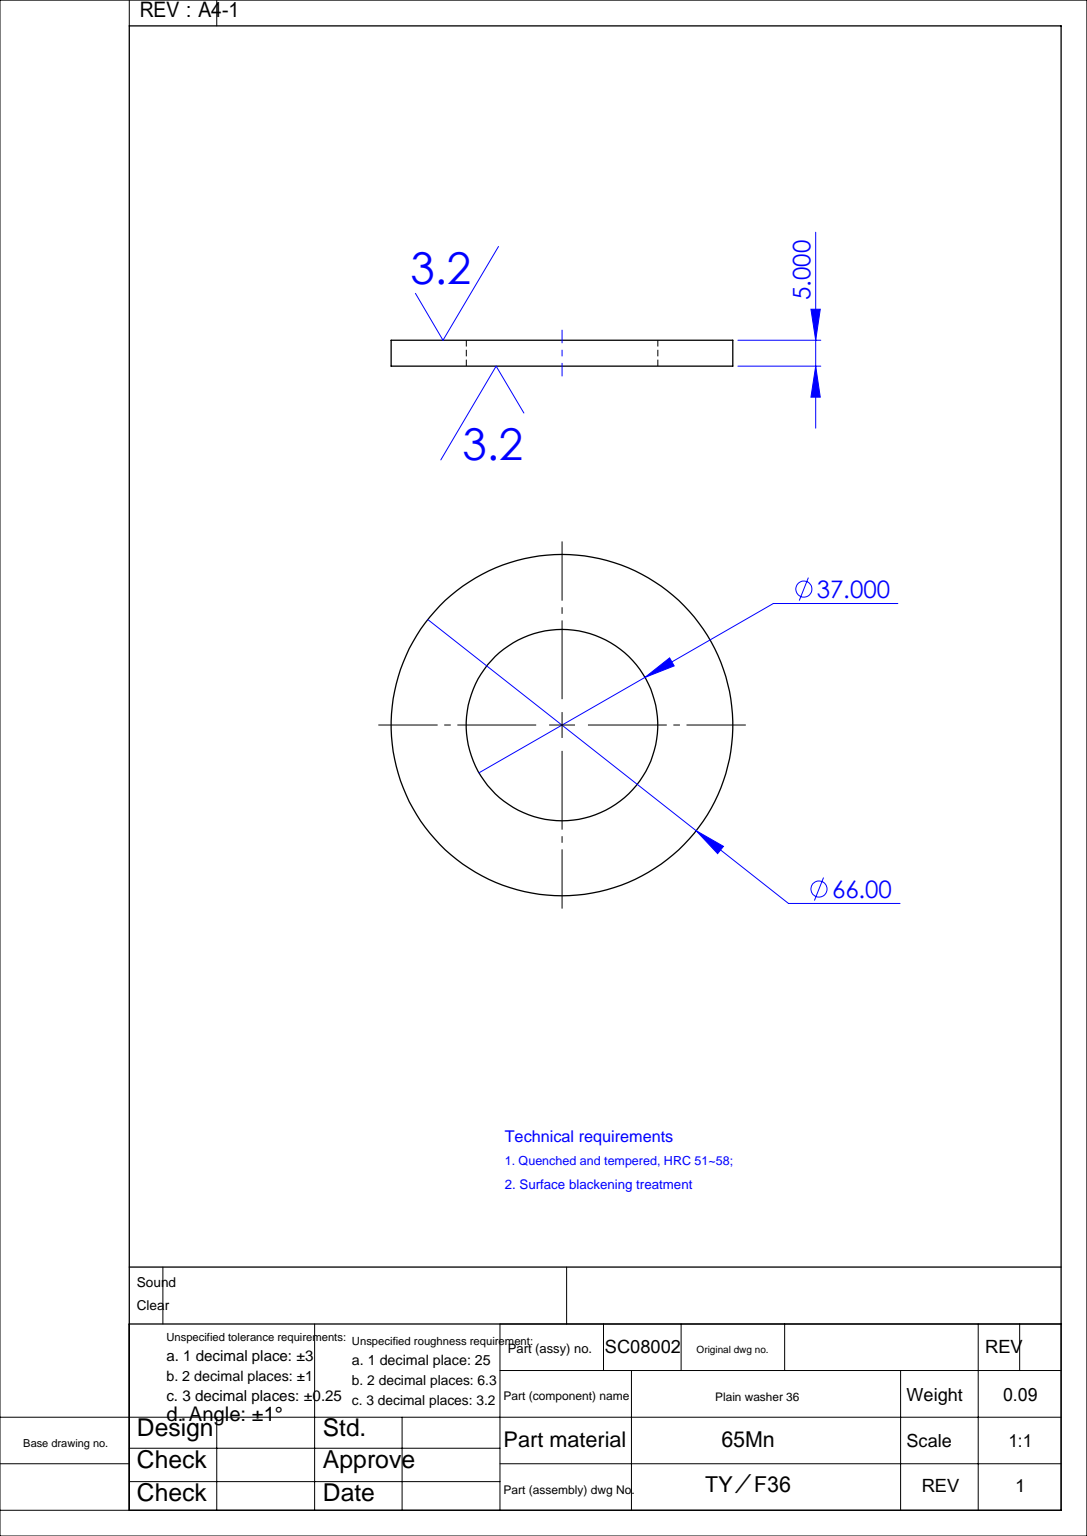
SolidWorks part; units mm, degrees
material "65Mn"
ref_plane "Plane1" through (0, 0, 0) normal (0, 0, 1) x (1, 0, 0)
ref_plane "Plane2" through (0, 0, 0) normal (0, 1, 0) x (1, 0, 0)
ref_plane "Plane3" through (0, 0, 0) normal (1, 0, 0) x (0, 0, -1)
sketch "Dimension sketch" plane through (0, 0, 0) normal (0, 0, 1) x (1, 0, 0)
  line L0 (0, 0) -> (9.1, 0)
  point P3 (1, 0)
  point P4 (10, 0)
  point P5 (5.5, 0)
  dimension "h" = 1
  dimension "d2" = 10
  dimension "d1" = 5.5
sketch "Sketch1" plane through (0, 0, 0) normal (0, 0, 1) x (1, 0, 0)
  line L0 (0, 0) -> (0, 52.7318) construction
  line L2 (-18.5, 8.6445) -> (-33, 8.6445)
  line L3 (-18.5, 8.6445) -> (-18.5, 13.6445)
  line L4 (-18.5, 13.6445) -> (-33, 13.6445)
  line L5 (-33, 8.6445) -> (-33, 13.6445)
  dimension "D1" = 37
  dimension "D2" = 66
  dimension "h" = 5
revolve "Base-Revolve" add sketch "Sketch1" angle 360 about L0
